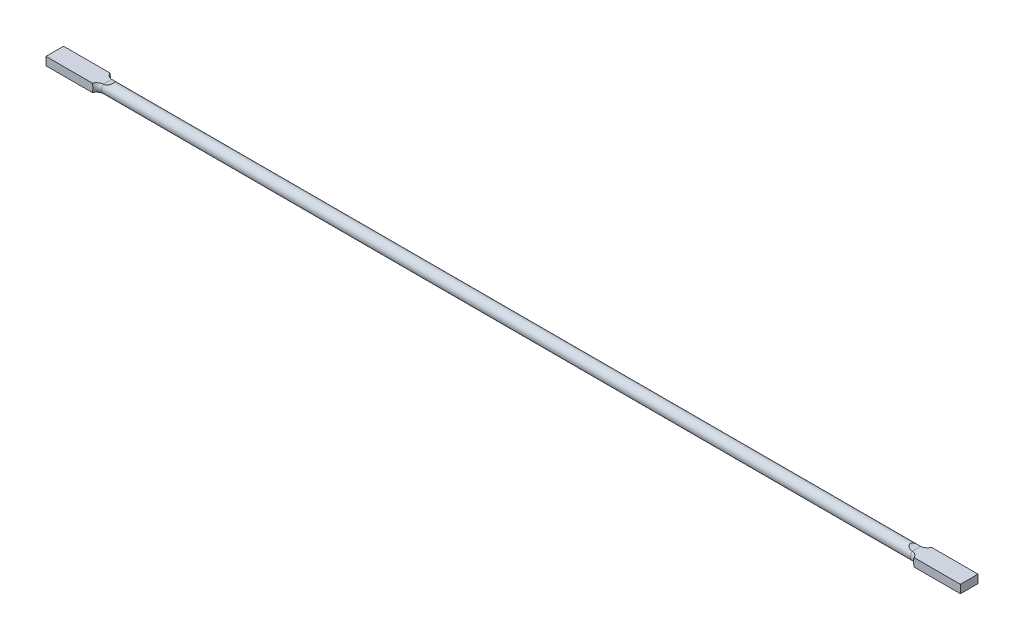
SolidWorks part; units mm, degrees
ref_plane "前视基准面" through (0, 0, 0) normal (0, 0, 1) x (1, 0, 0)
ref_plane "上视基准面" through (0, 0, 0) normal (0, 1, 0) x (1, 0, 0)
ref_plane "右视基准面" through (0, 0, 0) normal (1, 0, 0) x (0, 0, -1)
sketch "草图1" plane through (0, 0, 0) normal (0, 1, 0) x (1, 0, 0)
  line L0 (-32.4559, 0) -> (245.0195, 0) construction
  line L2 (0, -7.5) -> (45, -7.5)
  line L3 (0, -7.5) -> (0, 7.5)
  line L4 (0, 7.5) -> (45, 7.5)
  line L5 (45, -7.5) -> (45, 7.5)
  dimension "D1" = 7.5
extrude "凸台-拉伸1" add sketch "草图1" along normal mid plane 7
sketch "草图2" plane through (0, 0, 0) normal (0, 0, 1) x (1, 0, 0)
  line L0 (45, 3.5) -> (45, 0)
  line L1 (45, 0) -> (100, 0)
  line L2 (50, 5) -> (100, 5)
  line L3 (100, 5) -> (100, 0)
  line L7 (3.4681, 0) -> (112.0521, 0) construction
  line L8 (45, 3.5) -> (45, 5)
  line L9 (45, 5) -> (50, 5)
revolve "旋转1" add sketch "草图2" angle 360 about L7
sketch "草图3" plane through (0, 0, 0) normal (0, 0, 1) x (1, 0, 0)
  line L2 (100, 5) -> (45, 5) construction
  line L7 (45, -5) -> (100, -5) construction
  line L8 (50, -5) -> (50, -7.8721)
  line L9 (50, -7.8721) -> (45, -7.8721)
  line L10 (45, -7.8721) -> (45, -3.5)
  line L11 (45, 3.5) -> (45, 6.8777)
  line L12 (45, 6.8777) -> (50, 6.8777)
  line L13 (50, 6.8777) -> (50, 5)
  arc A0 (45, 3.5) -> (50, 5) centre (45, 12.5833) ccw
  arc A1 (45, -3.5) -> (50, -5) centre (45, -12.5833) cw
extrude "切除-拉伸1" cut sketch "草图3" against normal mid plane 10
sketch "草图4" plane through (0, 0, 0) normal (0, 1, 0) x (1, 0, 0)
  line L0 (45, 0) -> (-23.2609, 0) construction
  line L1 (45, -3.5707) -> (45, 3.5707) construction
  line L2 (45, 5) -> (40, 5) construction
  line L3 (40, 5) -> (40, 7.5) construction
  line L4 (45, 7.5) -> (0, 7.5) construction
  line L5 (45, 5) -> (51.8514, 5) construction
  line L6 (100, 5) -> (45, 5) construction
  line L8 (40, 11.25) -> (45, 11.25)
  line L9 (45, 11.25) -> (45, 5)
  line L10 (40, 11.25) -> (38.9196, 9.804)
  arc A0 (45, 5) -> (40, 7.5) centre (45, 11.25) cw
  arc A1 (40, 7.5) -> (38.9196, 9.804) centre (45, 11.25) cw
revolve "切除-旋转1" cut sketch "草图4" angle 360 about L0
sketch "草图5" plane through (100, 0, 0) normal (1, 0, 0) x (0, 0, -1)
  circle A0 centre (0, 0) radius 5
extrude "凸台-拉伸2" add sketch "草图5" along normal blind 290
mirror "镜向1" about plane through (390, 0, 0) normal (1, 0, 0) of bodies 120
